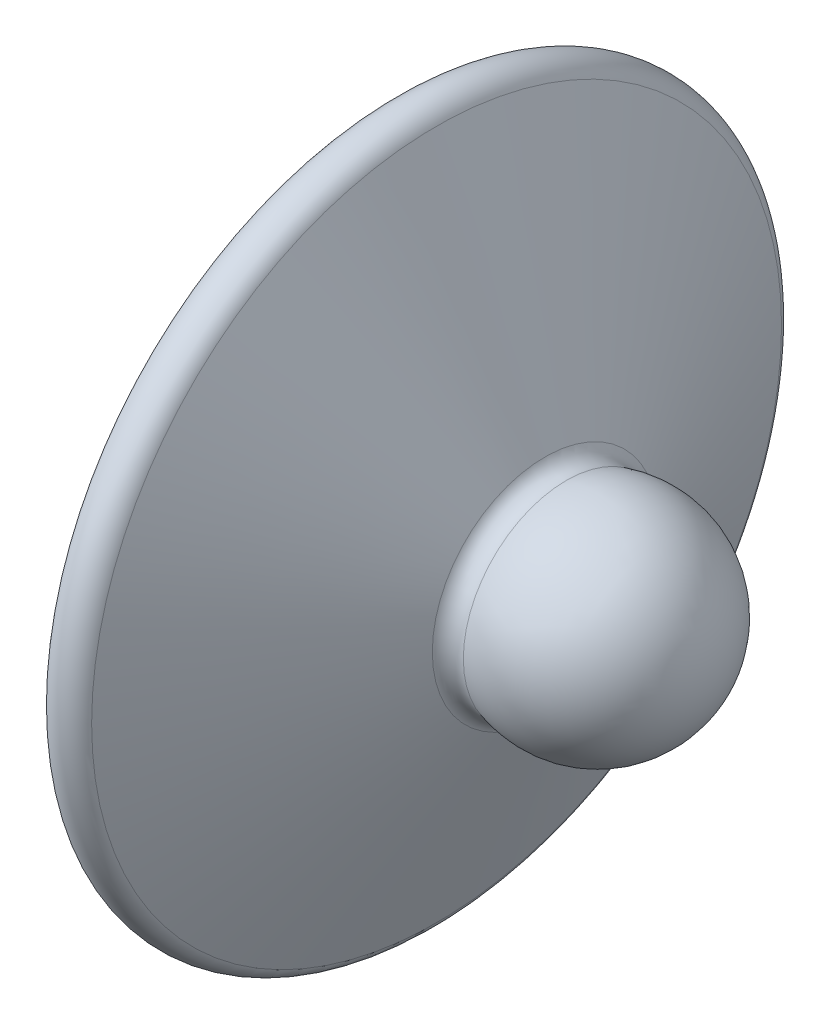
SolidWorks part; units mm, degrees
ref_plane "Front Plane" through (0, 0, 0) normal (0, 0, 1) x (1, 0, 0)
ref_plane "Top Plane" through (0, 0, 0) normal (0, 1, 0) x (1, 0, 0)
ref_plane "Right Plane" through (0, 0, 0) normal (1, 0, 0) x (0, 0, -1)
sketch "Sketch1" plane through (0, 0, 0) normal (0, 0, 1) x (1, 0, 0)
  line L0 (0, 0) -> (0, 6)
  line L1 (0, 6) -> (5, 6)
  line L2 (5, 6) -> (5, 18.6721)
  line L3 (7.5314, 19.2333) -> (13.572, 6.2791)
  line L4 (0, 0) -> (22.5, 0)
  line L5 (13.572, 6.2791) -> (16.5, 0) construction
  arc A1 (13.572, 6.2791) -> (14.7671, 5.7443) centre (14.4783, 6.7017) ccw
  arc A2 (14.7671, 5.7443) -> (22.5, 0) centre (16.5, 0) cw
  arc A3 (5, 18.6721) -> (7.5314, 19.2333) centre (6.3279, 18.6721) cw
  dimension "D3" = 6
  dimension "D5" = 20
  dimension "D7" = 1
  dimension "D1" = 6
  dimension "D2" = 5
  dimension "D4" = 16.5
  dimension "D6" = 65
revolve "Revolve1" add sketch "Sketch1" angle 360 about L4
chamfer "Chamfer1" distance 1 angle 45 1 edges at (0, 0, 6)
